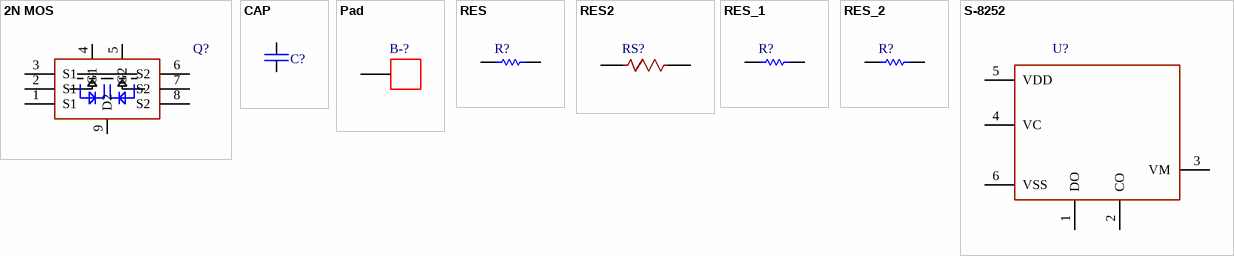
[diagram p0: symbols 2N MOS to S-8252]
# Altium schematic symbol library MISC78884.SCHLIB: 8 symbols
Pins are listed as number, name and electrical type; pins without a type are passive.


## 2N MOS
designator Q?
SMD MOS-TSSOP-8
footprint DFN3*3-L8(2N) (DFN3*3 dual SMD MOS)
pins: 1 S1, 2 S1, 3 S1, 4 G1, 5 G2, 6 S2, 7 S2, 8 S2, 9 D2

## CAP
designator C?
SMD capacitor
footprint C0402A (SMD capacitor)
footprint C0603A (SMD capacitor)
footprint C0402L (SMD resistor)
footprint C0805A (SMD capacitor)
footprint C1206A (SMD capacitor)
footprint C0603L (SMD J-type capacitor)
footprint C0805L (SMD capacitor)
pins: 1, 2

## Pad
designator B-?
Connection pad (non-through-hole)
footprint 3*3
footprint Pad10X8mm
footprint Pad8X6mm
pins: 1

## RES
designator R?
SMD resistor
footprint R0603A (SMD resistor)
footprint R0201A
footprint R0402A (SMD resistor)
footprint R0603m (SMD resistor)
footprint R0805A (SMD resistor)
footprint R0402L (SMD resistor)
footprint RES0603 (CAP0402)
footprint R0603L (SMD resistor)
footprint R0805L (SMD resistor)
pins: 1, 2

## RES2
designator RS?
SMD alloy resistor
footprint R2512L (SMD resistor)
pins: 1, 2

## RES_1
designator R?
SMD resistor
footprint R0603A (SMD resistor)
footprint R0201A
footprint R0402A (SMD resistor)
footprint R0603m (SMD resistor)
footprint R0805A (SMD resistor)
footprint R0402L (SMD resistor)
footprint RES0603 (CAP0402)
footprint R0603L (SMD resistor)
footprint R0805L (SMD resistor)
pins: 1, 2

## RES_2
designator R?
SMD resistor
footprint R0603A (SMD resistor)
footprint R0201A
footprint R0402A (SMD resistor)
footprint R0603m (SMD resistor)
footprint R0805A (SMD resistor)
footprint R0402L (SMD resistor)
footprint RES0603 (CAP0402)
footprint R0603L (SMD resistor)
footprint R0805L (SMD resistor)
pins: 1, 2

## S-8252
designator U?
2S battery protection IC
footprint SOT23-6A
footprint SOT23-6M (SMD MOS (special application)!!!)
pins: 1 DO, 2 CO, 3 VM, 4 VC, 5 VDD, 6 VSS